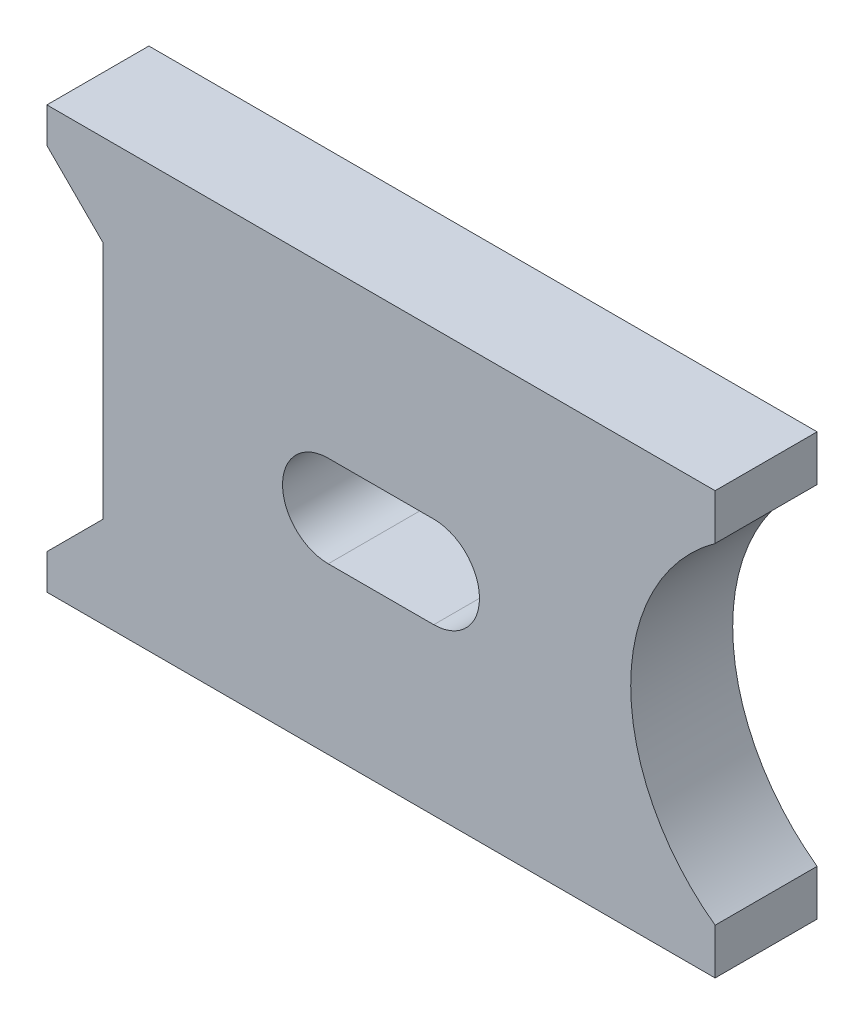
SolidWorks part; units mm, degrees
ref_plane "Front Plane" through (0, 0, 0) normal (0, 0, 1) x (1, 0, 0)
ref_plane "Top Plane" through (0, 0, 0) normal (0, 1, 0) x (1, 0, 0)
ref_plane "Right Plane" through (0, 0, 0) normal (1, 0, 0) x (0, 0, -1)
sketch "Sketch1" plane through (0, 0, 0) normal (0, 0, 1) x (1, 0, 0)
  line L0 (47.5, -23.5) -> (47.5, -30)
  line L1 (-47.5, 30) -> (47.5, 30)
  line L2 (-47.5, 30) -> (-47.5, 25)
  line L3 (-47.5, -30) -> (47.5, -30)
  line L4 (47.5, 30) -> (47.5, 23.5)
  line L5 (-47.5, 30) -> (47.5, -30) construction
  line L6 (-47.5, -30) -> (47.5, 30) construction
  line L7 (-39.5, 17) -> (-39.5, -17)
  line L8 (-39.5, 22) -> (-39.5, -22) construction
  line L9 (34.7485, -22) -> (34.7485, -22)
  line L10 (34.7485, 22) -> (34.7485, 22)
  line L12 (-39.5, -22) -> (34.7485, -22) construction
  line L13 (-39.5, 22) -> (34.7485, 22) construction
  line L14 (-47.5, -25) -> (-39.5, -17)
  line L15 (-47.5, -25) -> (-47.5, -30)
  line L16 (-47.5, 25) -> (-39.5, 17)
  line L17 (-47.5, 30) -> (-47.5, -30) construction
  line L19 (-7.5, 6.5) -> (7.5, 6.5)
  line L20 (-7.5, -6.5) -> (7.5, -6.5)
  arc A0 (47.5, 23.5) -> (47.5, -23.5) centre (64.5104, 0) ccw
  arc A1 (7.5, -6.5) -> (7.5, 6.5) centre (7.5, 0) ccw
  arc A2 (34.7485, 22) -> (34.7485, -22) centre (64.5104, 0) ccw construction
  arc A4 (-7.5, -6.5) -> (-7.5, 6.5) centre (-7.5, 0) cw
  point P0 (0, 0)
  point P6 (35.5, 0)
  point P7 (47.5, -23.5)
  point P8 (47.5, 0)
  point P9 (47.5, 23.5)
  point P20 (-39.5, 0)
  dimension "D1" = 12
  dimension "D2" = 23.5
  dimension "D3" = 23.5
  dimension "D5" = 95
  dimension "D4" = 8
extrude "Boss-Extrude1" add sketch "Sketch1" along normal blind 14.5 contours A0 L4 L1 L2 L16 L7 L14 L15 L3 L0 L20 A4 L19 A1
sketch "Sketch2" plane through (0, 0, 14.5) normal (0, 0, 1) x (1, 0, 0)
  line L0 (7.5, 0) -> (-7.5, 0)
